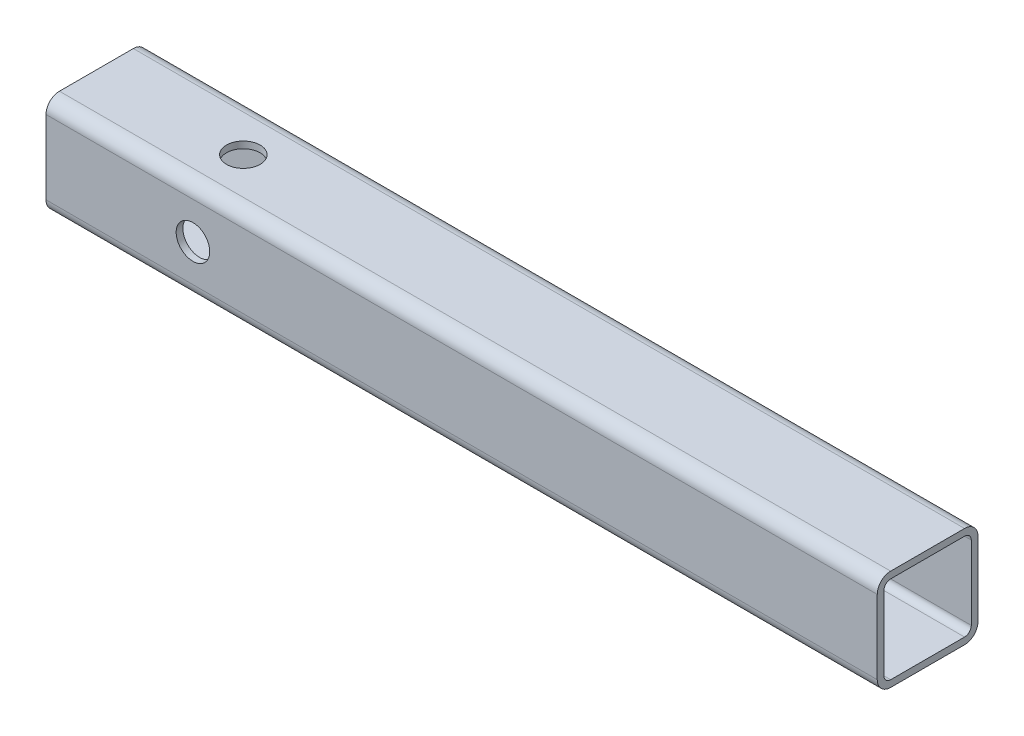
from build123d import *

# Parameters (mm, degrees)
GB_T6728_2002_60_X_60_X_4_1_DEPTH = 495
CUT_EXTRUDE_1_REACH               = 258.43
SKETCH_5_R                        = 10
CUT_EXTRUDE_2_REACH               = 258.43
SKETCH_6_R                        = 10


with BuildPart() as part:
    # Sketch1 → 冷弯空心方管gb∕t6728-2002 60 X 60 X 4(1) (new body)
    with BuildSketch(Plane.YZ.offset(-247.5)):
        with BuildLine():
            Line((-22, -30), (22, -30))
            ThreePointArc((22, -30), (27.656854249, -27.656854249), (30, -22))
            Line((30, -22), (30, 22))
            ThreePointArc((30, 22), (27.656854249, 27.656854249), (22, 30))
            Line((22, 30), (-22, 30))
            ThreePointArc((-22, 30), (-27.656854249, 27.656854249), (-30, 22))
            Line((-30, 22), (-30, -22))
            ThreePointArc((-30, -22), (-27.656854249, -27.656854249), (-22, -30))
        make_face()
        with BuildLine():
            Line((-22, -26), (22, -26))
            ThreePointArc((22, -26), (24.828427125, -24.828427125), (26, -22))
            Line((26, -22), (26, 22))
            ThreePointArc((26, 22), (24.828427125, 24.828427125), (22, 26))
            Line((22, 26), (-22, 26))
            ThreePointArc((-22, 26), (-24.828427125, 24.828427125), (-26, 22))
            Line((-26, 22), (-26, -22))
            ThreePointArc((-26, -22), (-24.828427125, -24.828427125), (-22, -26))
        make_face(mode=Mode.SUBTRACT)
    extrude(amount=GB_T6728_2002_60_X_60_X_4_1_DEPTH)

    # 切除-拉伸1: up to this face of the body (flat: up to its plane)
    cut_extrude_1_end = Plane(part.part.faces().sort_by_distance((0, 0, -30))[0])
    # 草图5 → 切除-拉伸1 (cut, up to the picked face)
    with BuildSketch(Plane.XY.offset(30), mode=Mode.PRIVATE) as cut_extrude_1_sk1:
        with Locations((-160, 0)):
            Circle(SKETCH_5_R)
    cut_extrude_1_tool1 = split(extrude(cut_extrude_1_sk1.sketch, amount=-CUT_EXTRUDE_1_REACH, mode=Mode.PRIVATE), bisect_by=cut_extrude_1_end, keep=Keep.BOTH, mode=Mode.PRIVATE)
    add(cut_extrude_1_tool1.solids().sort_by(Axis((-160, 0, 30), (0, 0, -1)))[0], mode=Mode.SUBTRACT)

    # 切除-拉伸2: up to this face of the body (flat: up to its plane)
    cut_extrude_2_end = Plane(part.part.faces().sort_by_distance((0, -30, 0))[0])
    # 草图6 → 切除-拉伸2 (cut, up to the picked face)
    with BuildSketch(Plane(origin=(0, 30, 0), x_dir=(1, 0, 0), z_dir=(0, 1, 0)), mode=Mode.PRIVATE) as cut_extrude_2_sk1:
        with Locations(Location((-160, 0, 0), (0, 0, 270))):
            Circle(SKETCH_6_R)
    cut_extrude_2_tool1 = split(extrude(cut_extrude_2_sk1.sketch, amount=-CUT_EXTRUDE_2_REACH, mode=Mode.PRIVATE), bisect_by=cut_extrude_2_end, keep=Keep.BOTH, mode=Mode.PRIVATE)
    add(cut_extrude_2_tool1.solids().sort_by(Axis((-160, 30, 0), (0, -1, 0)))[0], mode=Mode.SUBTRACT)


solid = part.part
